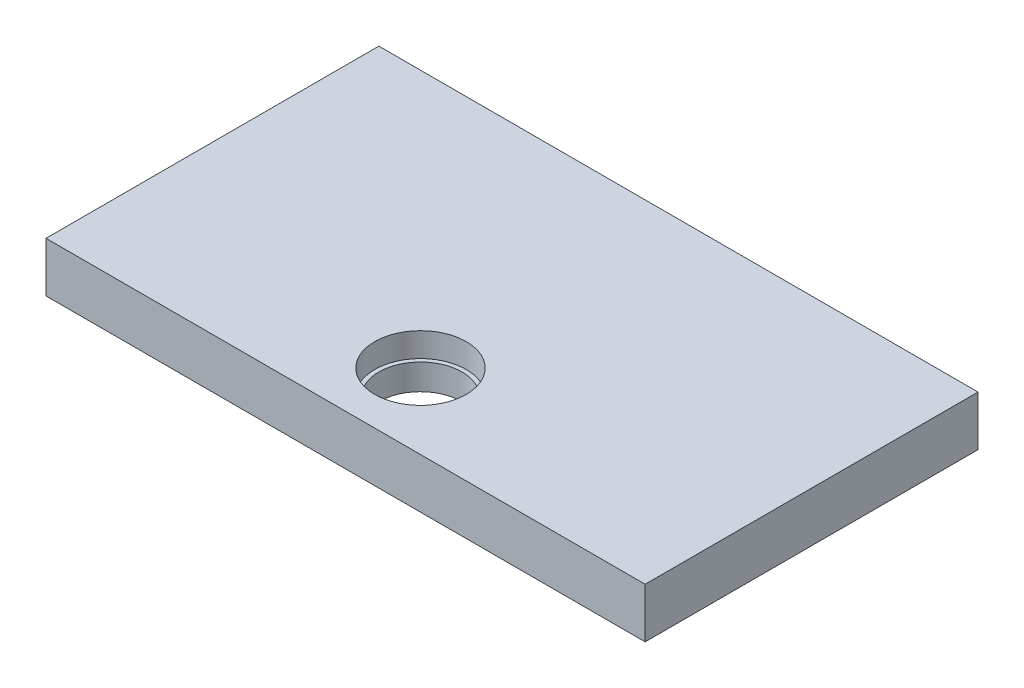
SolidWorks part; units mm, degrees
ref_plane "前视基准面" through (0, 0, 0) normal (0, 0, 1) x (1, 0, 0)
ref_plane "上视基准面" through (0, 0, 0) normal (0, 1, 0) x (1, 0, 0)
ref_plane "右视基准面" through (0, 0, 0) normal (1, 0, 0) x (0, 0, -1)
sketch "草图1" plane through (0, 0, 0) normal (0, 1, 0) x (1, 0, 0)
  line L1 (-180, -100) -> (180, -100)
  line L2 (-180, -100) -> (-180, 100)
  line L3 (-180, 100) -> (180, 100)
  line L4 (180, -100) -> (180, 100)
  line L5 (-180, -100) -> (180, 100) construction
  line L6 (-180, 100) -> (180, -100) construction
  point P0 (0, 0)
  dimension "D1" = 200
  dimension "D2" = 360
extrude "凸台-拉伸1" add sketch "草图1" along normal blind 30
sketch "草图2" plane through (0, 30, 0) normal (0, 1, 0) x (1, 0, 0)
  line L0 (180, -100) -> (180, 100) construction
  line L1 (180, 100) -> (-180, 100) construction
  circle A0 centre (0, -55) radius 27.5
  dimension "D1" = 55
  dimension "D2" = 180
  dimension "D3" = 155
extrude "切除-拉伸1" cut sketch "草图2" against normal blind 14.53
sketch "草图3" plane through (0, 30, 0) normal (0, 1, 0) x (1, 0, 0)
  line L0 (180, -100) -> (180, 100) construction
  line L1 (180, 100) -> (-180, 100) construction
  circle A0 centre (0, -55) radius 25
  dimension "D1" = 50
  dimension "D2" = 180
  dimension "D3" = 155
extrude "切除-拉伸2" cut sketch "草图3" against normal through all
